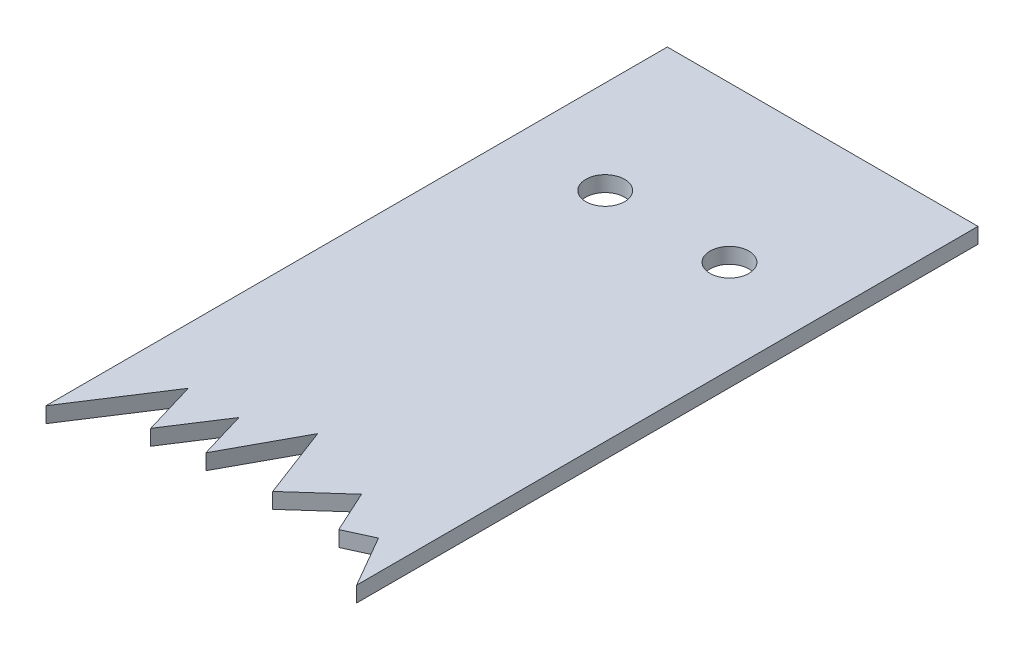
from build123d import *

# Parameters (mm, degrees)
SKETCH1_W           = 40
SKETCH1_H           = 80
BOSS_EXTRUDE1_DEPTH = 2
SKETCH2_R           = 2.5
CUT_EXTRUDE1_DEPTH  = 10
CUT_EXTRUDE2_DEPTH  = 10


with BuildPart() as part:
    # Sketch1 → Boss-Extrude1 (new body)
    with BuildSketch(Plane(origin=(0, 0, 0), x_dir=(1, 0, 0), z_dir=(0, 1, 0))):
        Rectangle(SKETCH1_W, SKETCH1_H)
    extrude(amount=BOSS_EXTRUDE1_DEPTH)

    # Sketch2 → Cut-Extrude1 (cut)
    with BuildSketch(Plane.XZ):
        with Locations(Location((8, -20, 0), (0, 0, 270))):
            Circle(SKETCH2_R)
        with Locations(Location((-8, -20, 0), (0, 0, 270))):
            Circle(SKETCH2_R)
    extrude(amount=-CUT_EXTRUDE1_DEPTH, mode=Mode.SUBTRACT)

    # Sketch3 → Cut-Extrude2 (cut)
    with BuildSketch(Plane(origin=(0, 2, 0), x_dir=(1, 0, 0), z_dir=(0, 1, 0))):
        Polygon((-20, -40), (-12.784626592, -28.891322442), (-10.73702175, -35.778720546), (-6.263478534, -28.891322442), (-4.459373627, -34.959675311), (0.603406691, -25.613003955), (4.154649825, -34.959675311), (10.180946182, -29.559865215), (12.65531235, -34.959675311), (16.161083178, -33.353218681), (20, -40), align=None)
    extrude(amount=-CUT_EXTRUDE2_DEPTH, mode=Mode.SUBTRACT)


solid = part.part
